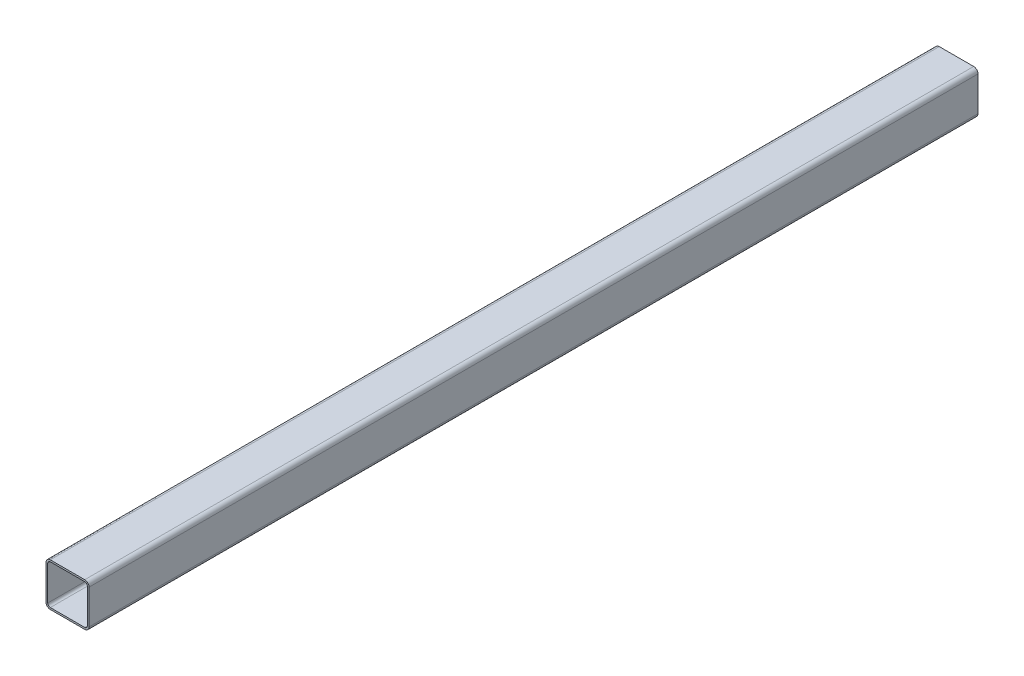
SolidWorks part; units mm, degrees
ref_plane "Front Plane" through (0, 0, 0) normal (0, 0, 1) x (1, 0, 0)
ref_plane "Top Plane" through (0, 0, 0) normal (0, 1, 0) x (1, 0, 0)
ref_plane "Right Plane" through (0, 0, 0) normal (1, 0, 0) x (0, 0, -1)
other "Configuration Table"
sketch "Sketch1" plane through (0, 0, 0) normal (0, 0, 1) x (1, 0, 0)
  line L0 (-92, 80) -> (-92, -80)
  line L1 (-80, 100) -> (80, 100)
  line L2 (-100, 80) -> (-100, -80)
  line L3 (-80, -100) -> (80, -100)
  line L4 (100, 80) -> (100, -80)
  line L5 (-100, 100) -> (100, -100) construction
  line L6 (-100, -100) -> (100, 100) construction
  line L7 (-80, -92) -> (80, -92)
  line L8 (92, 80) -> (92, -80)
  line L9 (-80, 92) -> (80, 92)
  arc A0 (-100, -80) -> (-80, -100) centre (-80, -80) ccw
  arc A1 (80, -100) -> (100, -80) centre (80, -80) ccw
  arc A2 (80, 100) -> (100, 80) centre (80, 80) cw
  arc A3 (-80, 100) -> (-100, 80) centre (-80, 80) ccw
  arc A4 (-92, -80) -> (-80, -92) centre (-80, -80) ccw
  arc A5 (80, -92) -> (92, -80) centre (80, -80) ccw
  arc A6 (80, 92) -> (92, 80) centre (80, 80) cw
  arc A7 (-80, 92) -> (-92, 80) centre (-80, 80) ccw
  point P0 (0, 0)
  dimension "D3" = 20
  dimension "D1" = 200
  dimension "D2" = 200
  dimension "D4" = 8
extrude "Boss-Extrude1" add sketch "Sketch1" along normal blind 4130
